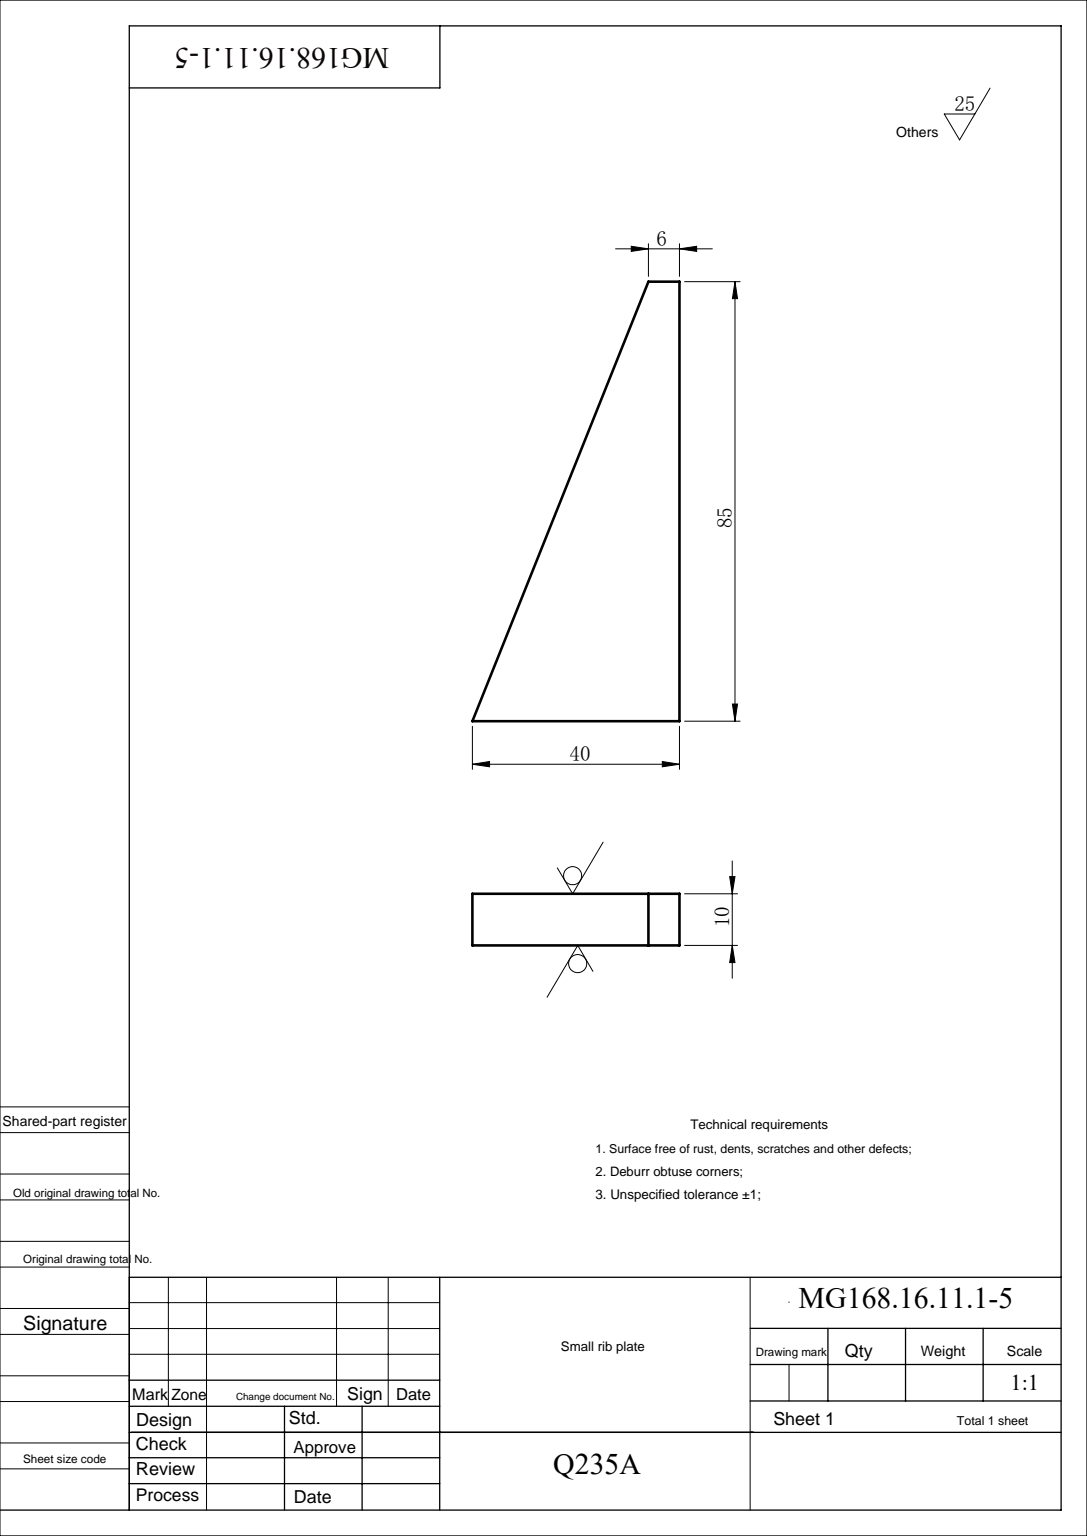
from build123d import *

# Parameters (mm, degrees)
BOSS_EXTRUDE1_DEPTH = 5


with BuildPart() as part:
    # Sketch1 → Boss-Extrude1 (new, symmetric)
    with BuildSketch(Plane(origin=(0, 0, 0), x_dir=(1, 0, 0), z_dir=(0, 1, 0))):
        Polygon((-6, 85), (-40, 0), (0, 0), (0, 85), align=None)
    extrude(amount=BOSS_EXTRUDE1_DEPTH, both=True)


solid = part.part
